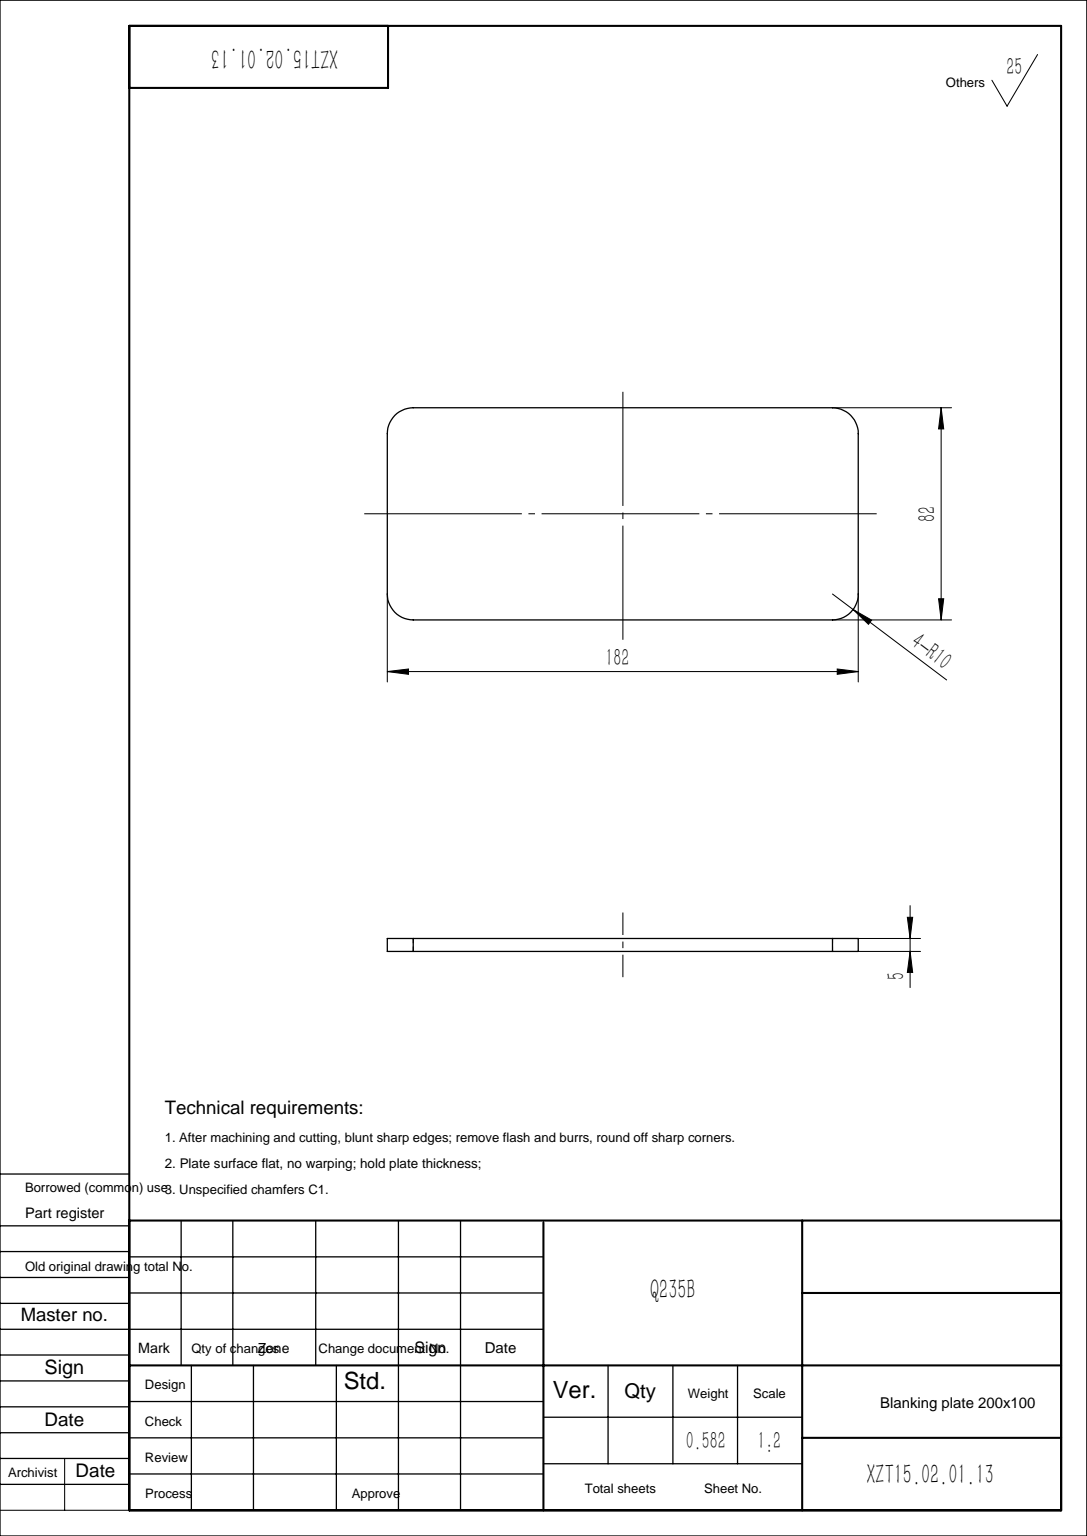
SolidWorks part; units mm, degrees
material "Q235B"
ref_plane "Front Plane" through (0, 0, 0) normal (0, 0, 1) x (1, 0, 0)
ref_plane "Top Plane" through (0, 0, 0) normal (0, 1, 0) x (1, 0, 0)
ref_plane "Right Plane" through (0, 0, 0) normal (1, 0, 0) x (0, 0, -1)
sketch "Sketch1" plane through (0, 0, 0) normal (0, 1, 0) x (1, 0, 0)
  line L1 (91, -41) -> (-91, -41)
  line L2 (91, -41) -> (91, 41)
  line L3 (91, 41) -> (-91, 41)
  line L4 (-91, -41) -> (-91, 41)
  line L5 (91, -41) -> (-91, 41) construction
  line L6 (91, 41) -> (-91, -41) construction
  point P0 (0, 0)
  dimension "D1" = 182
  dimension "D2" = 82
extrude "Boss-Extrude1" add sketch "Sketch1" along normal blind 5
hole_wizard "Ø9.0 (9) Diameter Hole1" positions "Sketch2" profile "Sketch3" hole size "Ø9.0" standard "GB"
sketch "Sketch2" plane through (0, 10, 0) normal (0, 1, 0) x (1, 0, 0)
  line L0 (-40, -30) -> (40, -30) construction
  line L1 (-40, -30) -> (-40, 30) construction
  line L2 (0, 0) -> (0, -30) construction
  line L4 (0, 0) -> (-40, 0) construction
  point P0 (-40, -30)
  point P8 (40, -30)
  point P9 (40, 30)
  point P10 (-40, 30)
  dimension "D3" = 90
  dimension "D4" = 80
  dimension "D5" = 60
  dimension "D1" = 2
  dimension "D2" = 2
sketch "Sketch3" plane through (-40, 10, 30) normal (1, 0, 0) x (0, 0, 1)
  line L0 (0, 0) -> (0, 10)
  line L1 (0, 10) -> (4.5, 10)
  line L2 (4.5, 10) -> (4.5, 0)
  line L5 (4.5, 0) -> (0, 0)
  line L11 (0, -6.35) -> (0, 107.95) construction
  dimension "通孔孔直径" = 9
  dimension "通孔孔深度" = 10
chamfer "Chamfer1" [suppressed] distance 10 angle 45
fillet "Fillet1" radius 10 4 edges at (91, 2.5, -41) (91, 2.5, 41) (-91, 2.5, 41) (-91, 2.5, -41)
